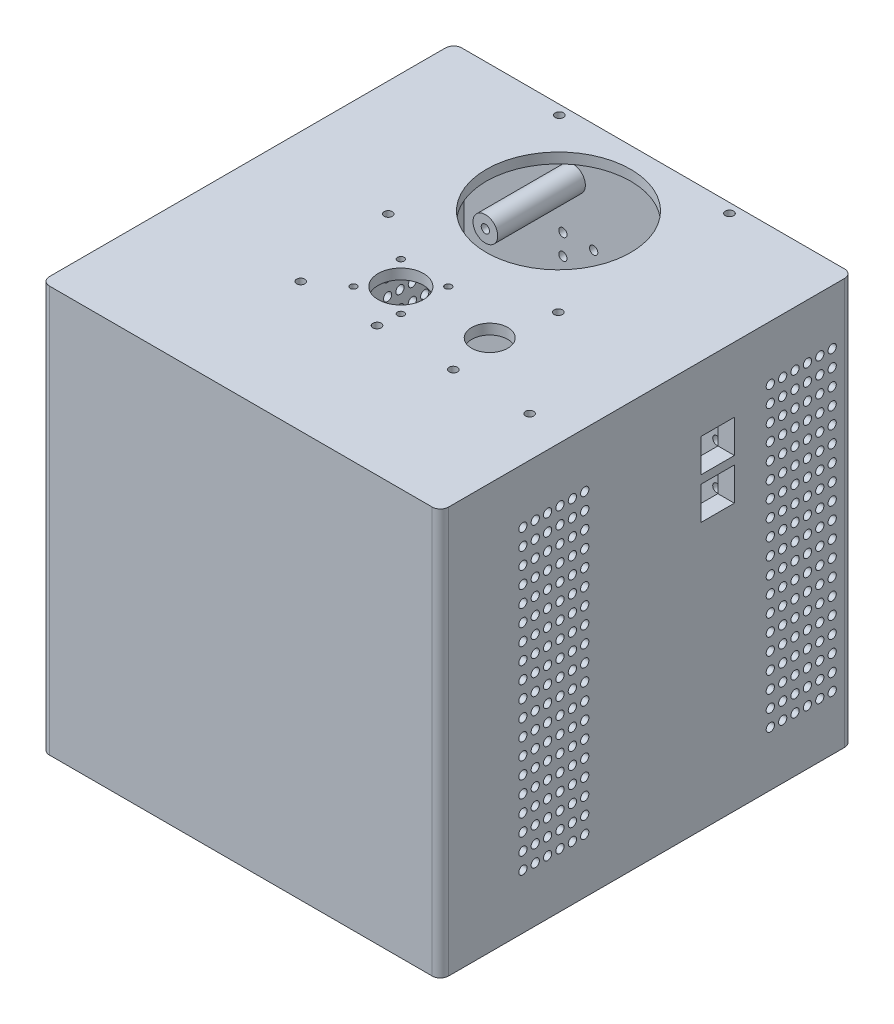
from build123d import *

# Parameters (mm, degrees)
SKETCH1_W                 = 183.595270985
SKETCH1_H                 = 195
BOSS_EXTRUDE1_DEPTH       = 200
SHELL2_T                  = -3
SKETCH4_W                 = 177.595270985
SKETCH4_H                 = 5
EXTRUDE_THIN1_DEPTH       = 170
SKETCH7_W                 = 15.113650162
SKETCH7_H                 = 15.232852339
SKETCH7_W_2               = 18.209612123
SKETCH7_H_2               = 17.140876259
CUT_EXTRUDE2_DEPTH        = 5
SKETCH8_W                 = 16.096108135
SKETCH8_H                 = 16.090598655
SKETCH8_W_2               = 16.049170695
SKETCH8_H_2               = 16.056481907
CUT_EXTRUDE3_DEPTH        = 5
SKETCH9_R                 = 2
SKETCH9_R_2               = 3
CUT_EXTRUDE4_DEPTH        = 5
BOSS_EXTRUDE3_START       = 46
SKETCH12_R                = 6
SKETCH12_R_2              = 2
BOSS_EXTRUDE3_DEPTH       = 46
CUT_EXTRUDE5_START        = 5
SKETCH15_R                = 4
CUT_EXTRUDE5_DEPTH        = 35
CUT_EXTRUDE6_DEPTH        = 335.263703575
CUT_EXTRUDE6_DEPTH_BACK   = 335.263703575
SKETCH16_W                = 41.839806916
SKETCH16_H                = 206.618939524
CHAMFER1_SIZE             = 4
CUT_EXTRUDE7_DEPTH        = 335.263703575
CUT_EXTRUDE7_DEPTH_BACK   = 30
SKETCH17_R                = 2
SKETCH19_W                = 183.595270985
SKETCH19_H                = 200
BOSS_EXTRUDE4_DEPTH       = 5
SKETCH20_R                = 8.75
SKETCH20_R_2              = 11
SKETCH20_R_3              = 1.6
CUT_EXTRUDE8_DEPTH        = 11
SURFACE_OFFSET1_1_D       = 5
THICKEN1_T2               = 5
SURFACE_OFFSET2_2_D       = 5
THICKEN2_T2               = 5
SKETCH21_R                = 2
CUT_EXTRUDE9_DEPTH        = 20
FILLET1_R                 = 4
CUT_EXTRUDE10_START       = -10
SKETCH22_R                = 2
CUT_EXTRUDE10_DEPTH       = 352.010452842
CUT_EXTRUDE11_DEPTH       = 319.290747588
CUT_EXTRUDE11_DEPTH_BACK  = 60
SKETCH23_R                = 2
SKETCH26_R                = 35
CUT_EXTRUDE12_DEPTH       = 5
LPATTERN1_COUNT           = 2
LPATTERN1_PITCH           = 120
LPATTERN1_START           = -10
LPATTERN1_COPY_1_SKETCH_R = 2
LPATTERN1_COPY_1_DEPTH    = 352.010452842
SKETCH28_W                = 54.114543349
SKETCH28_H                = 162.01509851
BOSS_EXTRUDE5_DEPTH       = 8
SKETCH29_W                = 13.954423589
SKETCH29_H                = 21.296250234
SKETCH29_W_2              = 23.479084835
CUT_EXTRUDE13_DEPTH       = 170
CUT_EXTRUDE14_DEPTH       = 10
SKETCH31_R                = 2
CUT_EXTRUDE15_DEPTH       = 15
SKETCH32_R                = 2
CUT_EXTRUDE16_DEPTH       = 10


with BuildPart() as part:
    # Sketch1 → Boss-Extrude1 (new body)
    with BuildSketch(Plane.XY):
        with Locations((-53.202364508, 97.5)):
            Rectangle(SKETCH1_W, SKETCH1_H)
    extrude(amount=BOSS_EXTRUDE1_DEPTH)

    # Shell2
    shell2_openings = [part.faces().sort_by_distance(p)[0] for p in [
        (-53.202364508, 0, 100),
    ]]
    offset(amount=SHELL2_T, openings=shell2_openings, kind=Kind.INTERSECTION)

    # Sketch4 → Extrude-Thin1 (add)
    with BuildSketch(Plane.XZ.offset(-192)):
        with Locations((-53.202364508, 48)):
            Rectangle(SKETCH4_W, SKETCH4_H)
    extrude(amount=EXTRUDE_THIN1_DEPTH)

    # Sketch7 → Cut-Extrude2 (cut)
    with BuildSketch(Plane.ZY.offset(145)):
        with Locations((64.970474072, 67.93327769)):
            Rectangle(SKETCH7_W, SKETCH7_H)
        with Locations((66.393347985, 122.87388666)):
            Rectangle(SKETCH7_W_2, SKETCH7_H_2)
    extrude(amount=-CUT_EXTRUDE2_DEPTH, mode=Mode.SUBTRACT)

    # Sketch8 → Cut-Extrude3 (cut)
    with BuildSketch(Plane(origin=(38.595270985, 0, 0), x_dir=(0, 0, -1), z_dir=(1, 0, 0))):
        with Locations((-65.447814288, 157.384866262)):
            Rectangle(SKETCH8_W, SKETCH8_H)
        with Locations((-65.473550459, 137.349026652)):
            Rectangle(SKETCH8_W_2, SKETCH8_H_2)
    extrude(amount=-CUT_EXTRUDE3_DEPTH, mode=Mode.SUBTRACT)

    # Sketch9 → Cut-Extrude4 (cut)
    with BuildSketch(Plane(origin=(0, 0, 45.5), x_dir=(-1, 0, 0), z_dir=(0, 0, -1))):
        with Locations((7.804729015, 172.226542544)):
            Circle(SKETCH9_R)
        with Locations(Location((7.804729015, 51.826542544, 0), (0, 0, 180))):
            Circle(SKETCH9_R_2)
        with Locations((89.104729015, 172.226542544)):
            Circle(SKETCH9_R)
        with Locations(Location((89.104729015, 51.826542544, 0), (0, 0, 180))):
            Circle(SKETCH9_R_2)
    extrude(amount=-CUT_EXTRUDE4_DEPTH, mode=Mode.SUBTRACT)

    # Sketch12 → Boss-Extrude3 (add)
    # profile 1 of 4: a face of its own
    with BuildSketch(Plane(origin=(0, 0, 45.5), x_dir=(-1, 0, 0), z_dir=(0, 0, -1)).offset(BOSS_EXTRUDE3_START)):
        with Locations(Location((7.704729015, 172.226542544, 0), (0, 0, 180))):
            Circle(SKETCH12_R)
        with Locations(Location((7.704729015, 172.226542544, 0), (0, 0, 180))):
            Circle(SKETCH12_R_2, mode=Mode.SUBTRACT)
    # profile 2 of 4: a face of its own
    with BuildSketch(Plane(origin=(0, 0, 45.5), x_dir=(-1, 0, 0), z_dir=(0, 0, -1)).offset(BOSS_EXTRUDE3_START)):
        with Locations(Location((89.104729015, 172.226542544, 0), (0, 0, 180))):
            Circle(SKETCH12_R)
        with Locations((89.104729015, 172.226542544)):
            Circle(SKETCH12_R_2, mode=Mode.SUBTRACT)
    # profile 3 of 4: a face of its own
    with BuildSketch(Plane(origin=(0, 0, 45.5), x_dir=(-1, 0, 0), z_dir=(0, 0, -1)).offset(BOSS_EXTRUDE3_START)):
        with Locations(Location((7.704729015, 51.826542544, 0), (0, 0, 180))):
            Circle(SKETCH12_R)
        with Locations(Location((7.704729015, 51.826542544, 0), (0, 0, 180))):
            Circle(SKETCH12_R_2, mode=Mode.SUBTRACT)
    # profile 4 of 4: a face of its own
    with BuildSketch(Plane(origin=(0, 0, 45.5), x_dir=(-1, 0, 0), z_dir=(0, 0, -1)).offset(BOSS_EXTRUDE3_START)):
        with Locations(Location((89.104729015, 51.826542544, 0), (0, 0, 180))):
            Circle(SKETCH12_R)
        with Locations(Location((89.104729015, 51.826542544, 0), (0, 0, 180))):
            Circle(SKETCH12_R_2, mode=Mode.SUBTRACT)
    extrude(amount=-BOSS_EXTRUDE3_DEPTH)

    # Sketch15 → Cut-Extrude5 (cut)
    with BuildSketch(Plane(origin=(0, 0, 0), x_dir=(-1, 0, 0), z_dir=(0, 0, -1)).offset(CUT_EXTRUDE5_START)):
        with Locations((89.104729015, 51.826542544)):
            Circle(SKETCH15_R)
        with Locations((7.704729015, 51.826542544)):
            Circle(SKETCH15_R)
        with Locations((7.704729015, 172.226542544)):
            Circle(SKETCH15_R)
        with Locations((89.104729015, 172.226542544)):
            Circle(SKETCH15_R)
    extrude(amount=-CUT_EXTRUDE5_DEPTH, mode=Mode.SUBTRACT)

    # Sketch16 → Cut-Extrude6 (cut, two sides: drawn at the far end of the back side and taken through both)
    with BuildSketch(Plane.ZY.offset(145).offset(-CUT_EXTRUDE6_DEPTH_BACK)):
        with Locations((-20.919903458, 103.309469762)):
            Rectangle(SKETCH16_W, SKETCH16_H)
    extrude(amount=CUT_EXTRUDE6_DEPTH + CUT_EXTRUDE6_DEPTH_BACK, mode=Mode.SUBTRACT)

    # Chamfer1
    chamfer1_edges = [part.edges().sort_by_distance(p)[0] for p in [
        (-3.704729015, 172.226542544, 0),
        (-85.104729015, 172.226542544, 0),
        (-3.704729015, 51.826542544, 0),
        (-85.104729015, 51.826542544, 0),
    ]]
    chamfer(chamfer1_edges, length=CHAMFER1_SIZE)

    # Sketch17 → Cut-Extrude7 (cut, two sides: drawn at the far end of the back side and taken through both)
    with BuildSketch(Plane.ZY.offset(145).offset(-CUT_EXTRUDE7_DEPTH_BACK)):
        with Locations(Location((188.225057207, 179.645787324, 0), (0, 0, 180))):
            Circle(SKETCH17_R)
        with Locations(Location((188.225057207, 99.645787324, 0), (0, 0, 180))):
            Circle(SKETCH17_R)
    extrude(amount=CUT_EXTRUDE7_DEPTH + CUT_EXTRUDE7_DEPTH_BACK, mode=Mode.SUBTRACT)

    # Sketch19 → Boss-Extrude4 (add)
    with BuildSketch(Plane.XZ.offset(-192)):
        with Locations((-53.202364508, 100)):
            Rectangle(SKETCH19_W, SKETCH19_H)
    extrude(amount=-BOSS_EXTRUDE4_DEPTH)

    # Sketch20 → Cut-Extrude8 (cut)
    with BuildSketch(Plane(origin=(0, 197, 0), x_dir=(1, 0, 0), z_dir=(0, 1, 0))):
        with Locations(Location((-17.487719836, -115, 0), (0, 0, 180))):
            Circle(SKETCH20_R)
        with Locations(Location((-60.587090294, -115, 0), (0, 0, 180))):
            Circle(SKETCH20_R_2)
        with Locations(Location((-49.087090294, -103.5, 0), (0, 0, 180))):
            Circle(SKETCH20_R_3)
        with Locations(Location((-49.087090294, -126.5, 0), (0, 0, 180))):
            Circle(SKETCH20_R_3)
        with Locations(Location((-72.087090294, -126.5, 0), (0, 0, 180))):
            Circle(SKETCH20_R_3)
        with Locations(Location((-72.087090294, -103.5, 0), (0, 0, 180))):
            Circle(SKETCH20_R_3)
    extrude(amount=-CUT_EXTRUDE8_DEPTH, mode=Mode.SUBTRACT)

    # Surface-Offset1: a surface, offset from 1 face of the part
    surface_offset1_1 = part.part.faces().sort_by_distance((-145, 98.458676303, 100.420701599))[0].offset(SURFACE_OFFSET1_1_D)
    add(Solid.thicken(surface_offset1_1, -THICKEN1_T2))

    # Surface-Offset2: a surface, offset from 1 face of the part
    surface_offset2_2 = part.part.faces().sort_by_distance((38.595270985, 97.850310558, 100.458965814))[0].offset(SURFACE_OFFSET2_2_D)
    add(Solid.thicken(surface_offset2_2, -THICKEN2_T2))

    # Sketch21 → Cut-Extrude9 (cut)
    with BuildSketch(Plane.XZ):
        with Locations((-146.109433088, 193.1642818)):
            Circle(SKETCH21_R)
        with Locations(Location((39.704704073, 193.1642818, 0), (0, 0, 180))):
            Circle(SKETCH21_R)
        with Locations((39.704704073, 6.8357182)):
            Circle(SKETCH21_R)
        with Locations(Location((-146.109433088, 6.8357182, 0), (0, 0, 180))):
            Circle(SKETCH21_R)
    extrude(amount=-CUT_EXTRUDE9_DEPTH, mode=Mode.SUBTRACT)

    # Fillet1
    fillet1_edges = [part.edges().sort_by_distance(p)[0] for p in [
        (-150, 98.5, 200),
        (-150, 98.5, 0),
        (43.595270985, 98.5, 200),
        (43.595270985, 98.5, 0),
    ]]
    fillet(fillet1_edges, radius=FILLET1_R)

    # Sketch22 → Cut-Extrude10 (cut)
    with BuildSketch(Plane.ZY.offset(150).offset(CUT_EXTRUDE10_START)):
        with Locations(Location((40, 170.5, 0), (0, 0, 180))):
            Circle(SKETCH22_R)
        with Locations(Location((34, 170.5, 0), (0, 0, 180))):
            Circle(SKETCH22_R)
        with Locations(Location((28, 170.5, 0), (0, 0, 180))):
            Circle(SKETCH22_R)
        with Locations(Location((34, 162.5, 0), (0, 0, 180))):
            Circle(SKETCH22_R)
        with Locations(Location((28, 162.5, 0), (0, 0, 180))):
            Circle(SKETCH22_R)
        with Locations(Location((34, 154.5, 0), (0, 0, 180))):
            Circle(SKETCH22_R)
        with Locations(Location((28, 154.5, 0), (0, 0, 180))):
            Circle(SKETCH22_R)
        with Locations(Location((34, 146.5, 0), (0, 0, 180))):
            Circle(SKETCH22_R)
        with Locations(Location((28, 146.5, 0), (0, 0, 180))):
            Circle(SKETCH22_R)
        with Locations(Location((34, 138.5, 0), (0, 0, 180))):
            Circle(SKETCH22_R)
        with Locations(Location((28, 138.5, 0), (0, 0, 180))):
            Circle(SKETCH22_R)
        with Locations(Location((34, 130.5, 0), (0, 0, 180))):
            Circle(SKETCH22_R)
        with Locations(Location((28, 130.5, 0), (0, 0, 180))):
            Circle(SKETCH22_R)
        with Locations(Location((34, 122.5, 0), (0, 0, 180))):
            Circle(SKETCH22_R)
        with Locations(Location((28, 122.5, 0), (0, 0, 180))):
            Circle(SKETCH22_R)
        with Locations(Location((34, 114.5, 0), (0, 0, 180))):
            Circle(SKETCH22_R)
        with Locations(Location((28, 114.5, 0), (0, 0, 180))):
            Circle(SKETCH22_R)
        with Locations(Location((34, 106.5, 0), (0, 0, 180))):
            Circle(SKETCH22_R)
        with Locations(Location((28, 106.5, 0), (0, 0, 180))):
            Circle(SKETCH22_R)
        with Locations(Location((34, 98.5, 0), (0, 0, 180))):
            Circle(SKETCH22_R)
        with Locations(Location((28, 98.5, 0), (0, 0, 180))):
            Circle(SKETCH22_R)
        with Locations(Location((34, 90.5, 0), (0, 0, 180))):
            Circle(SKETCH22_R)
        with Locations(Location((28, 90.5, 0), (0, 0, 180))):
            Circle(SKETCH22_R)
        with Locations(Location((34, 82.5, 0), (0, 0, 180))):
            Circle(SKETCH22_R)
        with Locations(Location((28, 82.5, 0), (0, 0, 180))):
            Circle(SKETCH22_R)
        with Locations(Location((34, 74.5, 0), (0, 0, 180))):
            Circle(SKETCH22_R)
        with Locations(Location((28, 74.5, 0), (0, 0, 180))):
            Circle(SKETCH22_R)
        with Locations(Location((34, 66.5, 0), (0, 0, 180))):
            Circle(SKETCH22_R)
        with Locations(Location((28, 66.5, 0), (0, 0, 180))):
            Circle(SKETCH22_R)
        with Locations(Location((34, 58.5, 0), (0, 0, 180))):
            Circle(SKETCH22_R)
        with Locations(Location((28, 58.5, 0), (0, 0, 180))):
            Circle(SKETCH22_R)
        with Locations(Location((34, 50.5, 0), (0, 0, 180))):
            Circle(SKETCH22_R)
        with Locations(Location((28, 50.5, 0), (0, 0, 180))):
            Circle(SKETCH22_R)
        with Locations(Location((34, 42.5, 0), (0, 0, 180))):
            Circle(SKETCH22_R)
        with Locations(Location((28, 42.5, 0), (0, 0, 180))):
            Circle(SKETCH22_R)
        with Locations(Location((34, 34.5, 0), (0, 0, 180))):
            Circle(SKETCH22_R)
        with Locations(Location((28, 34.5, 0), (0, 0, 180))):
            Circle(SKETCH22_R)
        with Locations(Location((34, 26.5, 0), (0, 0, 180))):
            Circle(SKETCH22_R)
        with Locations(Location((28, 26.5, 0), (0, 0, 180))):
            Circle(SKETCH22_R)
        with Locations(Location((40, 162.5, 0), (0, 0, 180))):
            Circle(SKETCH22_R)
        with Locations(Location((40, 154.5, 0), (0, 0, 180))):
            Circle(SKETCH22_R)
        with Locations(Location((40, 146.5, 0), (0, 0, 180))):
            Circle(SKETCH22_R)
        with Locations(Location((40, 138.5, 0), (0, 0, 180))):
            Circle(SKETCH22_R)
        with Locations(Location((40, 130.5, 0), (0, 0, 180))):
            Circle(SKETCH22_R)
        with Locations(Location((40, 122.5, 0), (0, 0, 180))):
            Circle(SKETCH22_R)
        with Locations(Location((40, 114.5, 0), (0, 0, 180))):
            Circle(SKETCH22_R)
        with Locations(Location((40, 106.5, 0), (0, 0, 180))):
            Circle(SKETCH22_R)
        with Locations(Location((40, 98.5, 0), (0, 0, 180))):
            Circle(SKETCH22_R)
        with Locations(Location((40, 90.5, 0), (0, 0, 180))):
            Circle(SKETCH22_R)
        with Locations(Location((40, 82.5, 0), (0, 0, 180))):
            Circle(SKETCH22_R)
        with Locations(Location((40, 74.5, 0), (0, 0, 180))):
            Circle(SKETCH22_R)
        with Locations(Location((40, 66.5, 0), (0, 0, 180))):
            Circle(SKETCH22_R)
        with Locations(Location((40, 58.5, 0), (0, 0, 180))):
            Circle(SKETCH22_R)
        with Locations(Location((40, 50.5, 0), (0, 0, 180))):
            Circle(SKETCH22_R)
        with Locations(Location((40, 42.5, 0), (0, 0, 180))):
            Circle(SKETCH22_R)
        with Locations(Location((40, 34.5, 0), (0, 0, 180))):
            Circle(SKETCH22_R)
        with Locations(Location((40, 26.5, 0), (0, 0, 180))):
            Circle(SKETCH22_R)
        with Locations(Location((22, 170.5, 0), (0, 0, 180))):
            Circle(SKETCH22_R)
        with Locations(Location((22, 162.5, 0), (0, 0, 180))):
            Circle(SKETCH22_R)
        with Locations(Location((22, 154.5, 0), (0, 0, 180))):
            Circle(SKETCH22_R)
        with Locations(Location((22, 146.5, 0), (0, 0, 180))):
            Circle(SKETCH22_R)
        with Locations(Location((22, 138.5, 0), (0, 0, 180))):
            Circle(SKETCH22_R)
        with Locations(Location((22, 130.5, 0), (0, 0, 180))):
            Circle(SKETCH22_R)
        with Locations(Location((22, 122.5, 0), (0, 0, 180))):
            Circle(SKETCH22_R)
        with Locations(Location((22, 114.5, 0), (0, 0, 180))):
            Circle(SKETCH22_R)
        with Locations(Location((22, 106.5, 0), (0, 0, 180))):
            Circle(SKETCH22_R)
        with Locations(Location((22, 98.5, 0), (0, 0, 180))):
            Circle(SKETCH22_R)
        with Locations(Location((22, 90.5, 0), (0, 0, 180))):
            Circle(SKETCH22_R)
        with Locations(Location((22, 82.5, 0), (0, 0, 180))):
            Circle(SKETCH22_R)
        with Locations(Location((22, 74.5, 0), (0, 0, 180))):
            Circle(SKETCH22_R)
        with Locations(Location((22, 66.5, 0), (0, 0, 180))):
            Circle(SKETCH22_R)
        with Locations(Location((22, 58.5, 0), (0, 0, 180))):
            Circle(SKETCH22_R)
        with Locations(Location((22, 50.5, 0), (0, 0, 180))):
            Circle(SKETCH22_R)
        with Locations(Location((22, 42.5, 0), (0, 0, 180))):
            Circle(SKETCH22_R)
        with Locations(Location((22, 34.5, 0), (0, 0, 180))):
            Circle(SKETCH22_R)
        with Locations(Location((22, 26.5, 0), (0, 0, 180))):
            Circle(SKETCH22_R)
        with Locations(Location((16, 170.5, 0), (0, 0, 180))):
            Circle(SKETCH22_R)
        with Locations(Location((16, 162.5, 0), (0, 0, 180))):
            Circle(SKETCH22_R)
        with Locations(Location((16, 154.5, 0), (0, 0, 180))):
            Circle(SKETCH22_R)
        with Locations(Location((16, 146.5, 0), (0, 0, 180))):
            Circle(SKETCH22_R)
        with Locations(Location((16, 138.5, 0), (0, 0, 180))):
            Circle(SKETCH22_R)
        with Locations(Location((16, 130.5, 0), (0, 0, 180))):
            Circle(SKETCH22_R)
        with Locations(Location((16, 122.5, 0), (0, 0, 180))):
            Circle(SKETCH22_R)
        with Locations(Location((16, 114.5, 0), (0, 0, 180))):
            Circle(SKETCH22_R)
        with Locations(Location((16, 106.5, 0), (0, 0, 180))):
            Circle(SKETCH22_R)
        with Locations(Location((16, 98.5, 0), (0, 0, 180))):
            Circle(SKETCH22_R)
        with Locations(Location((16, 90.5, 0), (0, 0, 180))):
            Circle(SKETCH22_R)
        with Locations(Location((16, 82.5, 0), (0, 0, 180))):
            Circle(SKETCH22_R)
        with Locations(Location((16, 74.5, 0), (0, 0, 180))):
            Circle(SKETCH22_R)
        with Locations(Location((16, 66.5, 0), (0, 0, 180))):
            Circle(SKETCH22_R)
        with Locations(Location((16, 58.5, 0), (0, 0, 180))):
            Circle(SKETCH22_R)
        with Locations(Location((16, 50.5, 0), (0, 0, 180))):
            Circle(SKETCH22_R)
        with Locations(Location((16, 42.5, 0), (0, 0, 180))):
            Circle(SKETCH22_R)
        with Locations(Location((16, 34.5, 0), (0, 0, 180))):
            Circle(SKETCH22_R)
        with Locations(Location((16, 26.5, 0), (0, 0, 180))):
            Circle(SKETCH22_R)
        with Locations(Location((10, 170.5, 0), (0, 0, 180))):
            Circle(SKETCH22_R)
        with Locations(Location((10, 162.5, 0), (0, 0, 180))):
            Circle(SKETCH22_R)
        with Locations(Location((10, 154.5, 0), (0, 0, 180))):
            Circle(SKETCH22_R)
        with Locations(Location((10, 146.5, 0), (0, 0, 180))):
            Circle(SKETCH22_R)
        with Locations(Location((10, 138.5, 0), (0, 0, 180))):
            Circle(SKETCH22_R)
        with Locations(Location((10, 130.5, 0), (0, 0, 180))):
            Circle(SKETCH22_R)
        with Locations(Location((10, 122.5, 0), (0, 0, 180))):
            Circle(SKETCH22_R)
        with Locations(Location((10, 114.5, 0), (0, 0, 180))):
            Circle(SKETCH22_R)
        with Locations(Location((10, 106.5, 0), (0, 0, 180))):
            Circle(SKETCH22_R)
        with Locations(Location((10, 98.5, 0), (0, 0, 180))):
            Circle(SKETCH22_R)
        with Locations(Location((10, 90.5, 0), (0, 0, 180))):
            Circle(SKETCH22_R)
        with Locations(Location((10, 82.5, 0), (0, 0, 180))):
            Circle(SKETCH22_R)
        with Locations(Location((10, 74.5, 0), (0, 0, 180))):
            Circle(SKETCH22_R)
        with Locations(Location((10, 66.5, 0), (0, 0, 180))):
            Circle(SKETCH22_R)
        with Locations(Location((10, 58.5, 0), (0, 0, 180))):
            Circle(SKETCH22_R)
        with Locations(Location((10, 50.5, 0), (0, 0, 180))):
            Circle(SKETCH22_R)
        with Locations(Location((10, 42.5, 0), (0, 0, 180))):
            Circle(SKETCH22_R)
        with Locations(Location((10, 34.5, 0), (0, 0, 180))):
            Circle(SKETCH22_R)
        with Locations(Location((10, 26.5, 0), (0, 0, 180))):
            Circle(SKETCH22_R)
    cut_extrude10 = extrude(amount=CUT_EXTRUDE10_DEPTH, mode=Mode.SUBTRACT)

    # Mirror1: Cut-Extrude10 across plane
    add(cut_extrude10.mirror(Plane.ZY.offset(53.202364508)), mode=Mode.SUBTRACT)

    # Sketch23 → Cut-Extrude11 (cut, two sides: drawn at the far end of the back side and taken through both)
    with BuildSketch(Plane(origin=(0, 0, 0), x_dir=(-1, 0, 0), z_dir=(0, 0, -1)).offset(-CUT_EXTRUDE11_DEPTH_BACK)):
        with Locations(Location((94, 77, 0), (0, 0, 180))):
            Circle(SKETCH23_R)
        with Locations(Location((79.067454836, 77, 0), (0, 0, 180))):
            Circle(SKETCH23_R)
        with Locations(Location((64.134909672, 77, 0), (0, 0, 180))):
            Circle(SKETCH23_R)
        with Locations(Location((49.202364508, 77, 0), (0, 0, 180))):
            Circle(SKETCH23_R)
        with Locations(Location((34.269819344, 77, 0), (0, 0, 180))):
            Circle(SKETCH23_R)
        with Locations(Location((19.337274179, 77, 0), (0, 0, 180))):
            Circle(SKETCH23_R)
        with Locations(Location((4.404729015, 77, 0), (0, 0, 180))):
            Circle(SKETCH23_R)
        with Locations(Location((79.067454836, 87, 0), (0, 0, 180))):
            Circle(SKETCH23_R)
        with Locations(Location((64.134909672, 87, 0), (0, 0, 180))):
            Circle(SKETCH23_R)
        with Locations(Location((49.202364508, 87, 0), (0, 0, 180))):
            Circle(SKETCH23_R)
        with Locations(Location((34.269819344, 87, 0), (0, 0, 180))):
            Circle(SKETCH23_R)
        with Locations(Location((19.337274179, 87, 0), (0, 0, 180))):
            Circle(SKETCH23_R)
        with Locations(Location((4.404729015, 87, 0), (0, 0, 180))):
            Circle(SKETCH23_R)
        with Locations(Location((79.067454836, 97, 0), (0, 0, 180))):
            Circle(SKETCH23_R)
        with Locations(Location((64.134909672, 97, 0), (0, 0, 180))):
            Circle(SKETCH23_R)
        with Locations(Location((49.202364508, 97, 0), (0, 0, 180))):
            Circle(SKETCH23_R)
        with Locations(Location((34.269819344, 97, 0), (0, 0, 180))):
            Circle(SKETCH23_R)
        with Locations(Location((19.337274179, 97, 0), (0, 0, 180))):
            Circle(SKETCH23_R)
        with Locations(Location((4.404729015, 97, 0), (0, 0, 180))):
            Circle(SKETCH23_R)
        with Locations(Location((79.067454836, 107, 0), (0, 0, 180))):
            Circle(SKETCH23_R)
        with Locations(Location((64.134909672, 107, 0), (0, 0, 180))):
            Circle(SKETCH23_R)
        with Locations(Location((49.202364508, 107, 0), (0, 0, 180))):
            Circle(SKETCH23_R)
        with Locations(Location((34.269819344, 107, 0), (0, 0, 180))):
            Circle(SKETCH23_R)
        with Locations(Location((19.337274179, 107, 0), (0, 0, 180))):
            Circle(SKETCH23_R)
        with Locations(Location((4.404729015, 107, 0), (0, 0, 180))):
            Circle(SKETCH23_R)
        with Locations(Location((79.067454836, 117, 0), (0, 0, 180))):
            Circle(SKETCH23_R)
        with Locations(Location((64.134909672, 117, 0), (0, 0, 180))):
            Circle(SKETCH23_R)
        with Locations(Location((49.202364508, 117, 0), (0, 0, 180))):
            Circle(SKETCH23_R)
        with Locations(Location((34.269819344, 117, 0), (0, 0, 180))):
            Circle(SKETCH23_R)
        with Locations(Location((19.337274179, 117, 0), (0, 0, 180))):
            Circle(SKETCH23_R)
        with Locations(Location((4.404729015, 117, 0), (0, 0, 180))):
            Circle(SKETCH23_R)
        with Locations(Location((79.067454836, 127, 0), (0, 0, 180))):
            Circle(SKETCH23_R)
        with Locations(Location((64.134909672, 127, 0), (0, 0, 180))):
            Circle(SKETCH23_R)
        with Locations(Location((49.202364508, 127, 0), (0, 0, 180))):
            Circle(SKETCH23_R)
        with Locations(Location((34.269819344, 127, 0), (0, 0, 180))):
            Circle(SKETCH23_R)
        with Locations(Location((19.337274179, 127, 0), (0, 0, 180))):
            Circle(SKETCH23_R)
        with Locations(Location((4.404729015, 127, 0), (0, 0, 180))):
            Circle(SKETCH23_R)
        with Locations(Location((79.067454836, 137, 0), (0, 0, 180))):
            Circle(SKETCH23_R)
        with Locations(Location((64.134909672, 137, 0), (0, 0, 180))):
            Circle(SKETCH23_R)
        with Locations(Location((49.202364508, 137, 0), (0, 0, 180))):
            Circle(SKETCH23_R)
        with Locations(Location((34.269819344, 137, 0), (0, 0, 180))):
            Circle(SKETCH23_R)
        with Locations(Location((19.337274179, 137, 0), (0, 0, 180))):
            Circle(SKETCH23_R)
        with Locations(Location((4.404729015, 137, 0), (0, 0, 180))):
            Circle(SKETCH23_R)
        with Locations(Location((79.067454836, 147, 0), (0, 0, 180))):
            Circle(SKETCH23_R)
        with Locations(Location((64.134909672, 147, 0), (0, 0, 180))):
            Circle(SKETCH23_R)
        with Locations(Location((49.202364508, 147, 0), (0, 0, 180))):
            Circle(SKETCH23_R)
        with Locations(Location((34.269819344, 147, 0), (0, 0, 180))):
            Circle(SKETCH23_R)
        with Locations(Location((19.337274179, 147, 0), (0, 0, 180))):
            Circle(SKETCH23_R)
        with Locations(Location((4.404729015, 147, 0), (0, 0, 180))):
            Circle(SKETCH23_R)
        with Locations(Location((94, 87, 0), (0, 0, 180))):
            Circle(SKETCH23_R)
        with Locations(Location((94, 97, 0), (0, 0, 180))):
            Circle(SKETCH23_R)
        with Locations(Location((94, 107, 0), (0, 0, 180))):
            Circle(SKETCH23_R)
        with Locations(Location((94, 117, 0), (0, 0, 180))):
            Circle(SKETCH23_R)
        with Locations(Location((94, 127, 0), (0, 0, 180))):
            Circle(SKETCH23_R)
        with Locations(Location((94, 137, 0), (0, 0, 180))):
            Circle(SKETCH23_R)
        with Locations(Location((94, 147, 0), (0, 0, 180))):
            Circle(SKETCH23_R)
    extrude(amount=CUT_EXTRUDE11_DEPTH + CUT_EXTRUDE11_DEPTH_BACK, mode=Mode.SUBTRACT)

    # Sketch26 → Cut-Extrude12 (cut)
    with BuildSketch(Plane(origin=(0, 197, 0), x_dir=(1, 0, 0), z_dir=(0, 1, 0))):
        with Locations(Location((-54.117613562, -45, 0), (0, 0, 180))):
            Circle(SKETCH26_R)
    extrude(amount=-CUT_EXTRUDE12_DEPTH, mode=Mode.SUBTRACT)

    # LPattern1: Cut-Extrude10 ×2
    with Locations(*[(0, 0, i * LPATTERN1_PITCH) for i in range(1, LPATTERN1_COUNT)]):
        add(cut_extrude10, mode=Mode.SUBTRACT)

    # LPattern1 copy 1 sketch → LPattern1 copy 1 (cut)
    with BuildSketch(Plane(origin=(43.595270985, 0, 120), x_dir=(0, 0, 1), z_dir=(1, 0, 0)).offset(LPATTERN1_START)):
        with Locations((40, -170.5)):
            Circle(LPATTERN1_COPY_1_SKETCH_R)
        with Locations((34, -170.5)):
            Circle(LPATTERN1_COPY_1_SKETCH_R)
        with Locations((28, -170.5)):
            Circle(LPATTERN1_COPY_1_SKETCH_R)
        with Locations((34, -162.5)):
            Circle(LPATTERN1_COPY_1_SKETCH_R)
        with Locations((28, -162.5)):
            Circle(LPATTERN1_COPY_1_SKETCH_R)
        with Locations((34, -154.5)):
            Circle(LPATTERN1_COPY_1_SKETCH_R)
        with Locations((28, -154.5)):
            Circle(LPATTERN1_COPY_1_SKETCH_R)
        with Locations((34, -146.5)):
            Circle(LPATTERN1_COPY_1_SKETCH_R)
        with Locations((28, -146.5)):
            Circle(LPATTERN1_COPY_1_SKETCH_R)
        with Locations((34, -138.5)):
            Circle(LPATTERN1_COPY_1_SKETCH_R)
        with Locations((28, -138.5)):
            Circle(LPATTERN1_COPY_1_SKETCH_R)
        with Locations((34, -130.5)):
            Circle(LPATTERN1_COPY_1_SKETCH_R)
        with Locations((28, -130.5)):
            Circle(LPATTERN1_COPY_1_SKETCH_R)
        with Locations((34, -122.5)):
            Circle(LPATTERN1_COPY_1_SKETCH_R)
        with Locations((28, -122.5)):
            Circle(LPATTERN1_COPY_1_SKETCH_R)
        with Locations((34, -114.5)):
            Circle(LPATTERN1_COPY_1_SKETCH_R)
        with Locations((28, -114.5)):
            Circle(LPATTERN1_COPY_1_SKETCH_R)
        with Locations((34, -106.5)):
            Circle(LPATTERN1_COPY_1_SKETCH_R)
        with Locations((28, -106.5)):
            Circle(LPATTERN1_COPY_1_SKETCH_R)
        with Locations((34, -98.5)):
            Circle(LPATTERN1_COPY_1_SKETCH_R)
        with Locations((28, -98.5)):
            Circle(LPATTERN1_COPY_1_SKETCH_R)
        with Locations((34, -90.5)):
            Circle(LPATTERN1_COPY_1_SKETCH_R)
        with Locations((28, -90.5)):
            Circle(LPATTERN1_COPY_1_SKETCH_R)
        with Locations((34, -82.5)):
            Circle(LPATTERN1_COPY_1_SKETCH_R)
        with Locations((28, -82.5)):
            Circle(LPATTERN1_COPY_1_SKETCH_R)
        with Locations((34, -74.5)):
            Circle(LPATTERN1_COPY_1_SKETCH_R)
        with Locations((28, -74.5)):
            Circle(LPATTERN1_COPY_1_SKETCH_R)
        with Locations((34, -66.5)):
            Circle(LPATTERN1_COPY_1_SKETCH_R)
        with Locations((28, -66.5)):
            Circle(LPATTERN1_COPY_1_SKETCH_R)
        with Locations((34, -58.5)):
            Circle(LPATTERN1_COPY_1_SKETCH_R)
        with Locations((28, -58.5)):
            Circle(LPATTERN1_COPY_1_SKETCH_R)
        with Locations((34, -50.5)):
            Circle(LPATTERN1_COPY_1_SKETCH_R)
        with Locations((28, -50.5)):
            Circle(LPATTERN1_COPY_1_SKETCH_R)
        with Locations((34, -42.5)):
            Circle(LPATTERN1_COPY_1_SKETCH_R)
        with Locations((28, -42.5)):
            Circle(LPATTERN1_COPY_1_SKETCH_R)
        with Locations((34, -34.5)):
            Circle(LPATTERN1_COPY_1_SKETCH_R)
        with Locations((28, -34.5)):
            Circle(LPATTERN1_COPY_1_SKETCH_R)
        with Locations((34, -26.5)):
            Circle(LPATTERN1_COPY_1_SKETCH_R)
        with Locations((28, -26.5)):
            Circle(LPATTERN1_COPY_1_SKETCH_R)
        with Locations((40, -162.5)):
            Circle(LPATTERN1_COPY_1_SKETCH_R)
        with Locations((40, -154.5)):
            Circle(LPATTERN1_COPY_1_SKETCH_R)
        with Locations((40, -146.5)):
            Circle(LPATTERN1_COPY_1_SKETCH_R)
        with Locations((40, -138.5)):
            Circle(LPATTERN1_COPY_1_SKETCH_R)
        with Locations((40, -130.5)):
            Circle(LPATTERN1_COPY_1_SKETCH_R)
        with Locations((40, -122.5)):
            Circle(LPATTERN1_COPY_1_SKETCH_R)
        with Locations((40, -114.5)):
            Circle(LPATTERN1_COPY_1_SKETCH_R)
        with Locations((40, -106.5)):
            Circle(LPATTERN1_COPY_1_SKETCH_R)
        with Locations((40, -98.5)):
            Circle(LPATTERN1_COPY_1_SKETCH_R)
        with Locations((40, -90.5)):
            Circle(LPATTERN1_COPY_1_SKETCH_R)
        with Locations((40, -82.5)):
            Circle(LPATTERN1_COPY_1_SKETCH_R)
        with Locations((40, -74.5)):
            Circle(LPATTERN1_COPY_1_SKETCH_R)
        with Locations((40, -66.5)):
            Circle(LPATTERN1_COPY_1_SKETCH_R)
        with Locations((40, -58.5)):
            Circle(LPATTERN1_COPY_1_SKETCH_R)
        with Locations((40, -50.5)):
            Circle(LPATTERN1_COPY_1_SKETCH_R)
        with Locations((40, -42.5)):
            Circle(LPATTERN1_COPY_1_SKETCH_R)
        with Locations((40, -34.5)):
            Circle(LPATTERN1_COPY_1_SKETCH_R)
        with Locations((40, -26.5)):
            Circle(LPATTERN1_COPY_1_SKETCH_R)
        with Locations((22, -170.5)):
            Circle(LPATTERN1_COPY_1_SKETCH_R)
        with Locations((22, -162.5)):
            Circle(LPATTERN1_COPY_1_SKETCH_R)
        with Locations((22, -154.5)):
            Circle(LPATTERN1_COPY_1_SKETCH_R)
        with Locations((22, -146.5)):
            Circle(LPATTERN1_COPY_1_SKETCH_R)
        with Locations((22, -138.5)):
            Circle(LPATTERN1_COPY_1_SKETCH_R)
        with Locations((22, -130.5)):
            Circle(LPATTERN1_COPY_1_SKETCH_R)
        with Locations((22, -122.5)):
            Circle(LPATTERN1_COPY_1_SKETCH_R)
        with Locations((22, -114.5)):
            Circle(LPATTERN1_COPY_1_SKETCH_R)
        with Locations((22, -106.5)):
            Circle(LPATTERN1_COPY_1_SKETCH_R)
        with Locations((22, -98.5)):
            Circle(LPATTERN1_COPY_1_SKETCH_R)
        with Locations((22, -90.5)):
            Circle(LPATTERN1_COPY_1_SKETCH_R)
        with Locations((22, -82.5)):
            Circle(LPATTERN1_COPY_1_SKETCH_R)
        with Locations((22, -74.5)):
            Circle(LPATTERN1_COPY_1_SKETCH_R)
        with Locations((22, -66.5)):
            Circle(LPATTERN1_COPY_1_SKETCH_R)
        with Locations((22, -58.5)):
            Circle(LPATTERN1_COPY_1_SKETCH_R)
        with Locations((22, -50.5)):
            Circle(LPATTERN1_COPY_1_SKETCH_R)
        with Locations((22, -42.5)):
            Circle(LPATTERN1_COPY_1_SKETCH_R)
        with Locations((22, -34.5)):
            Circle(LPATTERN1_COPY_1_SKETCH_R)
        with Locations((22, -26.5)):
            Circle(LPATTERN1_COPY_1_SKETCH_R)
        with Locations((16, -170.5)):
            Circle(LPATTERN1_COPY_1_SKETCH_R)
        with Locations((16, -162.5)):
            Circle(LPATTERN1_COPY_1_SKETCH_R)
        with Locations((16, -154.5)):
            Circle(LPATTERN1_COPY_1_SKETCH_R)
        with Locations((16, -146.5)):
            Circle(LPATTERN1_COPY_1_SKETCH_R)
        with Locations((16, -138.5)):
            Circle(LPATTERN1_COPY_1_SKETCH_R)
        with Locations((16, -130.5)):
            Circle(LPATTERN1_COPY_1_SKETCH_R)
        with Locations((16, -122.5)):
            Circle(LPATTERN1_COPY_1_SKETCH_R)
        with Locations((16, -114.5)):
            Circle(LPATTERN1_COPY_1_SKETCH_R)
        with Locations((16, -106.5)):
            Circle(LPATTERN1_COPY_1_SKETCH_R)
        with Locations((16, -98.5)):
            Circle(LPATTERN1_COPY_1_SKETCH_R)
        with Locations((16, -90.5)):
            Circle(LPATTERN1_COPY_1_SKETCH_R)
        with Locations((16, -82.5)):
            Circle(LPATTERN1_COPY_1_SKETCH_R)
        with Locations((16, -74.5)):
            Circle(LPATTERN1_COPY_1_SKETCH_R)
        with Locations((16, -66.5)):
            Circle(LPATTERN1_COPY_1_SKETCH_R)
        with Locations((16, -58.5)):
            Circle(LPATTERN1_COPY_1_SKETCH_R)
        with Locations((16, -50.5)):
            Circle(LPATTERN1_COPY_1_SKETCH_R)
        with Locations((16, -42.5)):
            Circle(LPATTERN1_COPY_1_SKETCH_R)
        with Locations((16, -34.5)):
            Circle(LPATTERN1_COPY_1_SKETCH_R)
        with Locations((16, -26.5)):
            Circle(LPATTERN1_COPY_1_SKETCH_R)
        with Locations((10, -170.5)):
            Circle(LPATTERN1_COPY_1_SKETCH_R)
        with Locations((10, -162.5)):
            Circle(LPATTERN1_COPY_1_SKETCH_R)
        with Locations((10, -154.5)):
            Circle(LPATTERN1_COPY_1_SKETCH_R)
        with Locations((10, -146.5)):
            Circle(LPATTERN1_COPY_1_SKETCH_R)
        with Locations((10, -138.5)):
            Circle(LPATTERN1_COPY_1_SKETCH_R)
        with Locations((10, -130.5)):
            Circle(LPATTERN1_COPY_1_SKETCH_R)
        with Locations((10, -122.5)):
            Circle(LPATTERN1_COPY_1_SKETCH_R)
        with Locations((10, -114.5)):
            Circle(LPATTERN1_COPY_1_SKETCH_R)
        with Locations((10, -106.5)):
            Circle(LPATTERN1_COPY_1_SKETCH_R)
        with Locations((10, -98.5)):
            Circle(LPATTERN1_COPY_1_SKETCH_R)
        with Locations((10, -90.5)):
            Circle(LPATTERN1_COPY_1_SKETCH_R)
        with Locations((10, -82.5)):
            Circle(LPATTERN1_COPY_1_SKETCH_R)
        with Locations((10, -74.5)):
            Circle(LPATTERN1_COPY_1_SKETCH_R)
        with Locations((10, -66.5)):
            Circle(LPATTERN1_COPY_1_SKETCH_R)
        with Locations((10, -58.5)):
            Circle(LPATTERN1_COPY_1_SKETCH_R)
        with Locations((10, -50.5)):
            Circle(LPATTERN1_COPY_1_SKETCH_R)
        with Locations((10, -42.5)):
            Circle(LPATTERN1_COPY_1_SKETCH_R)
        with Locations((10, -34.5)):
            Circle(LPATTERN1_COPY_1_SKETCH_R)
        with Locations((10, -26.5)):
            Circle(LPATTERN1_COPY_1_SKETCH_R)
    extrude(amount=LPATTERN1_COPY_1_DEPTH, mode=Mode.SUBTRACT)

    # Sketch28 → Boss-Extrude5 (add)
    with BuildSketch(Plane(origin=(-142, 0, 0), x_dir=(0, 0, -1), z_dir=(1, 0, 0))):
        with Locations((-143.617637171, 97.253729166)):
            Rectangle(SKETCH28_W, SKETCH28_H)
    extrude(amount=-BOSS_EXTRUDE5_DEPTH)

    # Sketch29 → Cut-Extrude13 (cut)
    with BuildSketch(Plane.XZ.offset(-22)):
        with Locations((28.61805919, 39.851874883)):
            Rectangle(SKETCH29_W, SKETCH29_H)
        with Locations((-130.260457583, 39.851874883)):
            Rectangle(SKETCH29_W_2, SKETCH29_H)
    extrude(amount=-CUT_EXTRUDE13_DEPTH, mode=Mode.SUBTRACT)

    # Sketch30 → Cut-Extrude14 (cut)
    with BuildSketch(Plane(origin=(0, 0, 45.5), x_dir=(-1, 0, 0), z_dir=(0, 0, -1))):
        Polygon((-21.640847396, 22), (118.520915165, 22), (118.520915165, 192), (89.114041951, 192), (19.121185172, 192), (-21.640847396, 192), align=None)
    extrude(amount=-CUT_EXTRUDE14_DEPTH, mode=Mode.SUBTRACT)

    # Sketch31 → Cut-Extrude15 (cut)
    with BuildSketch(Plane(origin=(0, 197, 0), x_dir=(1, 0, 0), z_dir=(0, 1, 0))):
        with Locations(Location((-86.986809063, -137.154967319, 0), (0, 0, 180))):
            Circle(SKETCH31_R)
        with Locations(Location((-49.986809063, -137.154967319, 0), (0, 0, 180))):
            Circle(SKETCH31_R)
        with Locations(Location((-12.986809063, -137.154967319, 0), (0, 0, 180))):
            Circle(SKETCH31_R)
        with Locations(Location((24.013190937, -137.154967319, 0), (0, 0, 180))):
            Circle(SKETCH31_R)
    extrude(amount=-CUT_EXTRUDE15_DEPTH, mode=Mode.SUBTRACT)

    # Sketch32 → Cut-Extrude16 (cut)
    with BuildSketch(Plane(origin=(0, 197, 0), x_dir=(1, 0, 0), z_dir=(0, 1, 0))):
        with Locations(Location((-11.631233886, -87.581563216, 0), (0, 0, 180))):
            Circle(SKETCH32_R)
        with Locations(Location((-94.131233886, -87.581563216, 0), (0, 0, 180))):
            Circle(SKETCH32_R)
        with Locations(Location((-11.631233886, -4.581563216, 0), (0, 0, 180))):
            Circle(SKETCH32_R)
        with Locations(Location((-94.131233886, -4.581563216, 0), (0, 0, 180))):
            Circle(SKETCH32_R)
    extrude(amount=-CUT_EXTRUDE16_DEPTH, mode=Mode.SUBTRACT)


solid = part.part
